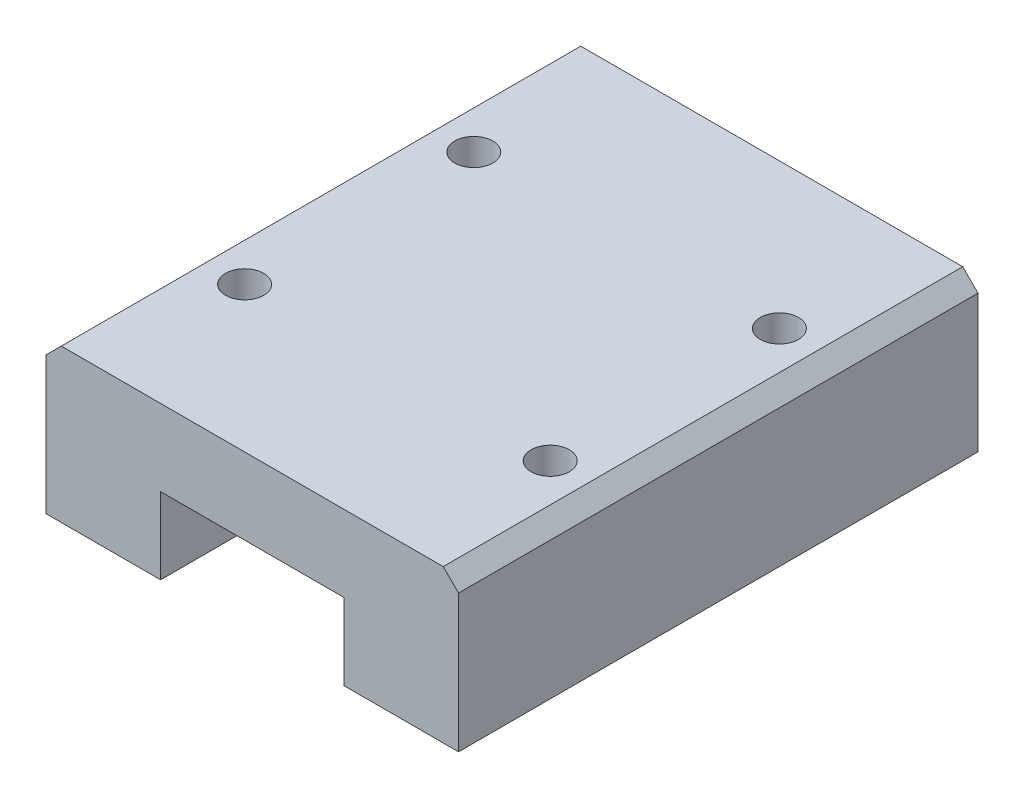
SolidWorks part; units mm, degrees
ref_plane "前视基准面" through (0, 0, 0) normal (0, 0, 1) x (1, 0, 0)
ref_plane "上视基准面" through (0, 0, 0) normal (0, 1, 0) x (1, 0, 0)
ref_plane "右视基准面" through (0, 0, 0) normal (1, 0, 0) x (0, 0, -1)
sketch "草图1" plane through (0, 0, 0) normal (0, 0, 1) x (1, 0, 0)
  line L0 (-6, 0) -> (6, 0)
  line L1 (13.5, 5) -> (-13.5, 5)
  line L2 (13.5, 5) -> (13.5, -5)
  line L3 (13.5, -5) -> (6, -5)
  line L4 (-13.5, 5) -> (-13.5, -5)
  line L5 (13.5, 5) -> (-13.5, -5) construction
  line L6 (13.5, -5) -> (-13.5, 5) construction
  line L7 (-6, 0) -> (-6, -5)
  line L8 (6, 0) -> (6, -5)
  line L9 (-6, -5) -> (-13.5, -5)
  point P0 (0, 0)
  point P8 (0, 0)
  dimension "D1" = 27
  dimension "D2" = 10
  dimension "D3" = 12
  dimension "D4" = 5
extrude "凸台-拉伸1" add sketch "草图1" along normal blind 34
hole_wizard "M3 螺纹孔1" positions "草图3" profile "草图2" tap size "M3" standard "Iso"
sketch "草图3" plane through (0, 5, 0) normal (0, 1, 0) x (1, 0, 0)
  line L0 (-10, -9.5) -> (10, -9.5) construction
  line L1 (-10, -9.5) -> (-10, -24.5) construction
  line L2 (-10, -24.5) -> (10, -24.5) construction
  line L3 (10, -24.5) -> (10, -9.5) construction
  line L5 (-15.317, -17) -> (16.653, -17) construction
  line L7 (-13.5, -34) -> (-13.5, 0) construction
  point P0 (-10, -9.5)
  point P2 (10, -9.5)
  point P9 (0, -9.5)
  point P11 (-10, -24.5)
  point P13 (10, -24.5)
  point P27 (10, -17)
  point P31 (-13.5, -17)
  dimension "D1" = 20
  dimension "D2" = 15
sketch "草图2" plane through (-10, 5, 9.5) normal (1, 0, 0) x (0, 0, 1)
  line L0 (0, 0) -> (0, 8.2511)
  line L1 (0, 8.2511) -> (1.25, 7.5)
  line L2 (1.25, 7.5) -> (1.25, 0)
  line L5 (1.25, 0) -> (0, 0)
  line L10 (0, 8.2511) -> (-1.25, 7.5) construction
  line L11 (0, -6.35) -> (0, 107.95) construction
  dimension "螺纹孔钻头直径" = 2.5
  dimension "螺纹孔钻头深度" = 7.5
  dimension "导头角度" = 118
chamfer "倒角1" distance 1 distance2 1 2 edges at (-13.5, 5, 17) (13.5, 5, 17)
